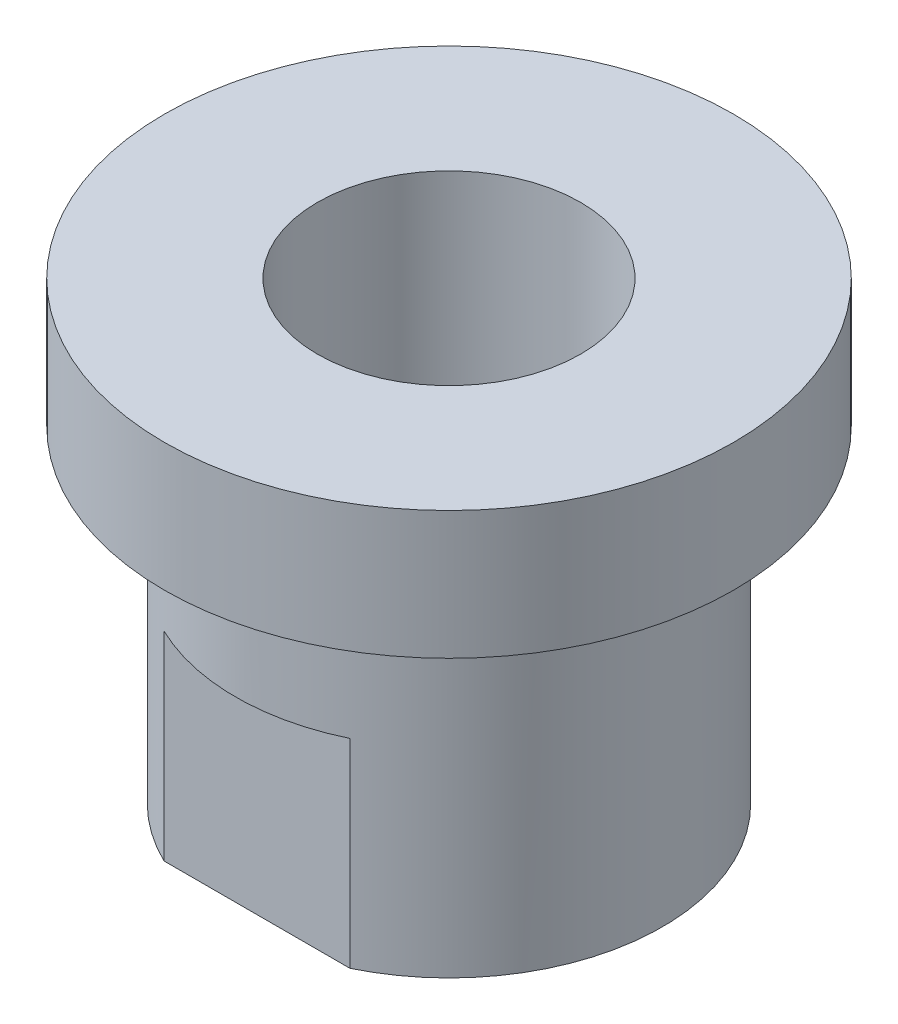
SolidWorks part; units mm, degrees
material "45#"
ref_plane "Front" through (0, 0, 0) normal (0, 0, 1) x (1, 0, 0)
ref_plane "Top" through (0, 0, 0) normal (0, 1, 0) x (1, 0, 0)
ref_plane "Right" through (0, 0, 0) normal (1, 0, 0) x (0, 0, -1)
sketch "Sketch1" plane through (0, 0, 0) normal (0, 1, 0) x (1, 0, 0)
  circle A0 centre (0, 0) radius 20
  circle A1 centre (0, 0) radius 9
  dimension "D1" = 40
  dimension "D2" = 18
extrude "Boss-Extrude1" add sketch "Sketch1" along normal blind 32
sketch "Sketch2" plane through (0, 0, 0) normal (0, -1, 0) x (1, 0, 0)
  circle A0 centre (0, 0) radius 15
  circle A1 centre (0, 0) radius 25
  dimension "D1" = 30
  dimension "D2" = 50
extrude "Cut-Extrude1" cut sketch "Sketch2" against normal blind 23
sketch "Sketch3" plane through (0, 0, 0) normal (1, 0, 0) x (0, 0, -1)
  line L0 (0, 0) -> (0, 13.5863) construction
  line L1 (-20.9887, 14) -> (-13.5, 14)
  line L2 (-20.9887, 14) -> (-20.9887, -7.2902)
  line L3 (-20.9887, -7.2902) -> (-13.5, -7.2902)
  line L4 (-13.5, 14) -> (-13.5, -7.2902)
  line L5 (13.5, 14) -> (13.5, -7.2902)
  line L6 (20.9887, -7.2902) -> (13.5, -7.2902)
  line L7 (20.9887, 14) -> (20.9887, -7.2902)
  line L8 (20.9887, 14) -> (13.5, 14)
  line L9 (-15, 0) -> (15, 0) construction
  dimension "D1" = 27
  dimension "D2" = 14
extrude "Cut-Extrude2" cut sketch "Sketch3" against normal through all both and the other way through all
hole_wizard "M20x1.5 Tapped Hole1" positions "Sketch4" profile "Sketch5" tap size "M20x1.5" standard "GB" end condition through all
sketch "Sketch4" plane through (0, 32, 0) normal (0, 1, 0) x (1, 0, 0)
  point P0 (0, 0)
sketch "Sketch5" plane through (0, 32, 0) normal (1, 0, 0) x (0, 0, 1)
  line L0 (0, 0) -> (0, 32)
  line L1 (0, 32) -> (9.25, 32)
  line L2 (9.25, 32) -> (9.25, 0)
  line L5 (9.25, 0) -> (0, 0)
  line L11 (0, -6.35) -> (0, 107.95) construction
  dimension "通孔螺纹孔钻头直径" = 18.5
  dimension "通孔螺纹孔钻头深度" = 32
cosmetic thread "Hole Thread1" parameters "D2"=20
